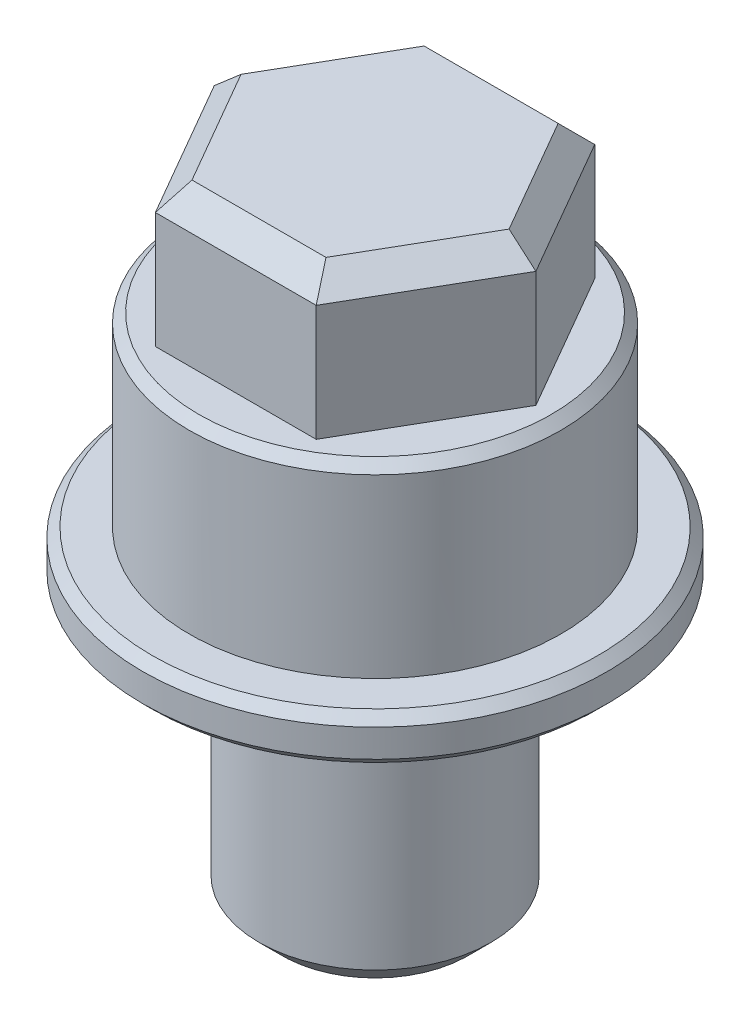
SolidWorks part; units mm, degrees
material "SUS304"
ref_plane "Front Plane" through (0, 0, 0) normal (0, 0, 1) x (1, 0, 0)
ref_plane "Top Plane" through (0, 0, 0) normal (0, 1, 0) x (1, 0, 0)
ref_plane "Right Plane" through (0, 0, 0) normal (1, 0, 0) x (0, 0, -1)
sketch "Sketch2" plane through (0, 0, 0) normal (0, 0, 1) x (1, 0, 0)
  line L0 (0, 0) -> (0, 14.0706) construction
  line L1 (0, 0) -> (2.5, 0)
  line L2 (2.5, 0) -> (2.5, 6)
  line L3 (2.5, 6) -> (5, 6)
  line L4 (5, 6) -> (5, 7)
  line L5 (4, 14) -> (0, 14)
  line L6 (0, 14) -> (0, 0)
  line L8 (5, 7) -> (4, 7)
  line L11 (4, 7) -> (4, 14)
  dimension "D1" = 1
  dimension "D2" = 6
  dimension "D3" = 2.5
  dimension "D4" = 5
  dimension "D5" = 4
  dimension "D6" = 14
revolve "Revolve1" add sketch "Sketch2" angle 360 about L0
cosmetic thread "Cosmetic Thread1" parameters "D1"=6, "D2"=4.134
sketch "Sketch4" plane through (0, 14, 0) normal (0, 1, 0) x (1, 0, 0)
  line L1 (1.7321, 3) -> (-1.7321, 3)
  line L2 (-1.7321, 3) -> (-3.4641, 0)
  line L3 (-3.4641, 0) -> (-1.7321, -3)
  line L4 (-1.7321, -3) -> (1.7321, -3)
  line L5 (1.7321, -3) -> (3.4641, 0)
  line L6 (3.4641, 0) -> (1.7321, 3)
  circle A0 centre (0, 0) radius 3 construction
  dimension "D1" = 6
extrude "Cut-Extrude2" cut sketch "Sketch4" against normal blind 3 flip side to cut
chamfer "Chamfer1" distance 0.5 angle 45 7 edges at (0, 0, -2.5) (0, 14, 3) (-2.5981, 14, 1.5) (-2.5981, 14, -1.5) (0, 14, -3) (2.5981, 14, -1.5) (2.5981, 14, 1.5)
chamfer "Chamfer2" distance 0.2 angle 45 3 edges at (0, 6, -5) (0, 7, -5) (0, 11, 4)
